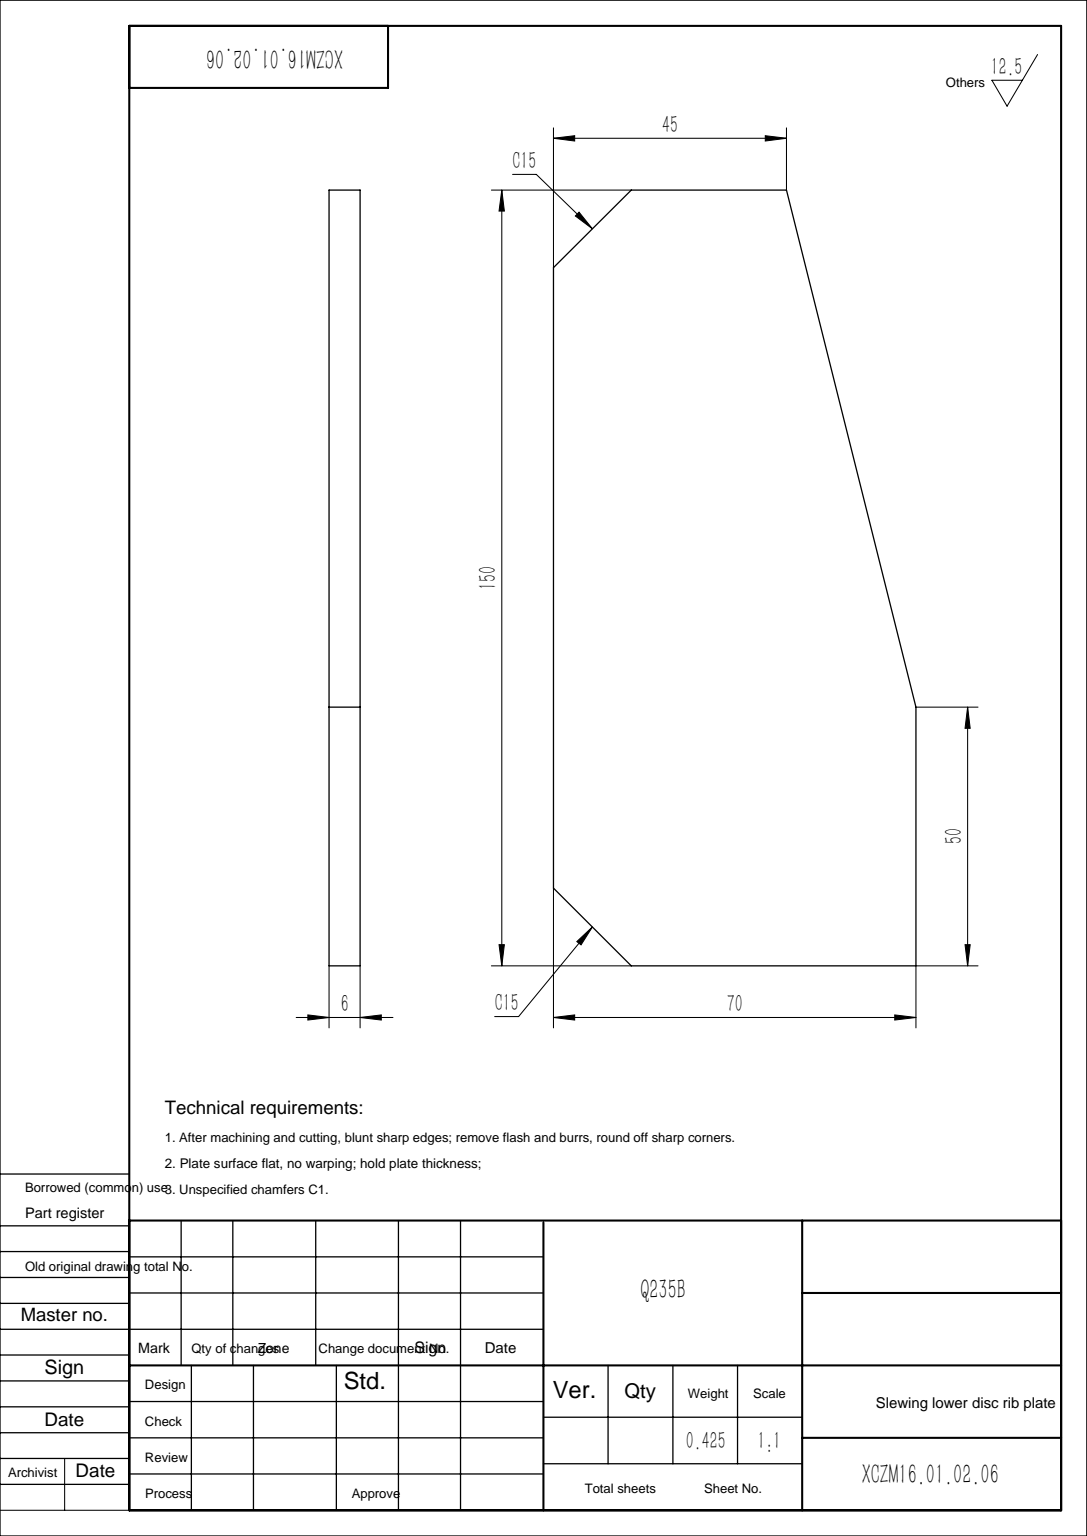
from build123d import *

# Parameters (mm, degrees)
BOSS_EXTRUDE1_DEPTH = 6
CHAMFER1_SIZE       = 15


with BuildPart() as part:
    # Sketch1 → Boss-Extrude1 (new body)
    with BuildSketch(Plane.XY):
        Polygon((0, 150), (0, 0), (70, 0), (70, 50), (45, 150), align=None)
    extrude(amount=BOSS_EXTRUDE1_DEPTH)

    # Chamfer1
    chamfer1_edges = [part.edges().sort_by_distance(p)[0] for p in [
        (0, 0, 3),
        (0, 150, 3),
    ]]
    chamfer(chamfer1_edges, length=CHAMFER1_SIZE)


solid = part.part
